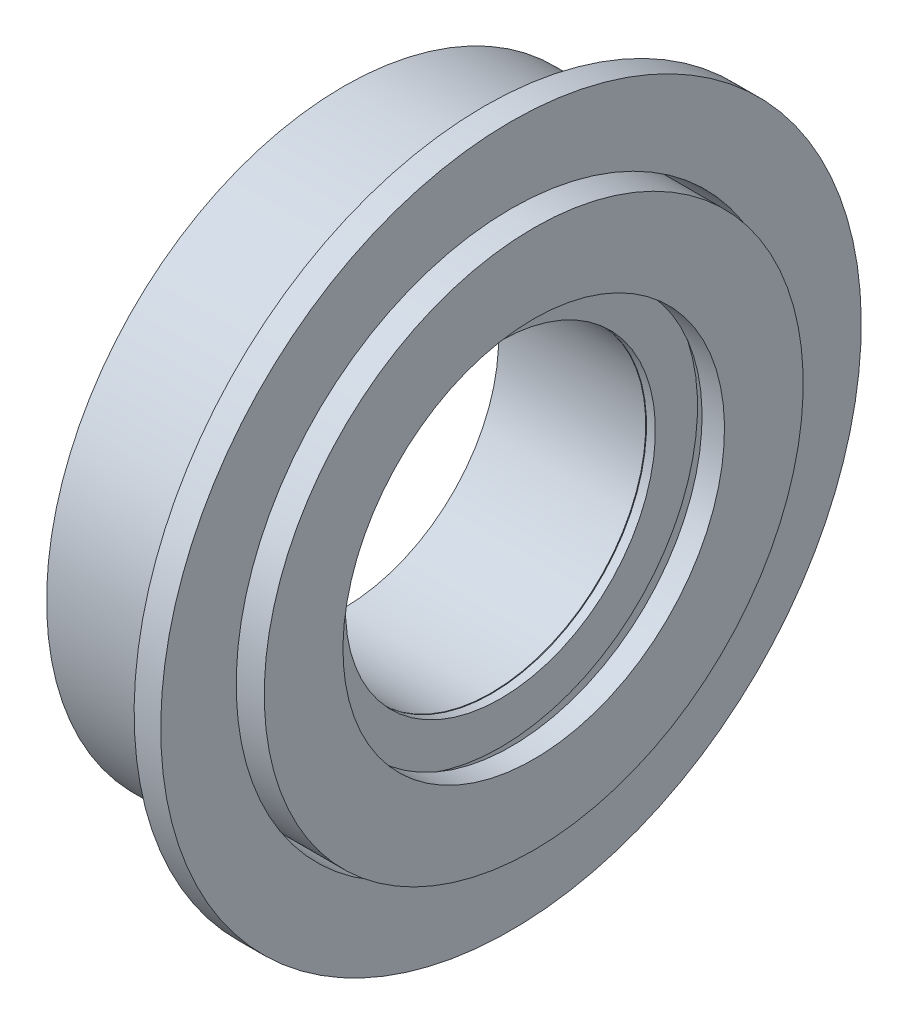
from build123d import *

# Parameters (mm, degrees)
SKETCH1_W   = 12.624761142
SKETCH1_H   = 6.080044682
SKETCH1_W_2 = 1
SKETCH1_H_2 = 4.744556516


with BuildPart() as part:
    # Sketch1 → Revolve1 (revolve)
    with BuildSketch(Plane.XY):
        Polygon((93, 39.45458405), (93, 33.45458405), (93, 30.95458405), (77, 30.95458405), (77, 20.45458405), (90.724333667, 20.45458405), (90.724333667, 17.45458405), (74.14259961, 17.45458405), (74.14259961, 33.45458405), (90, 33.45458405), (90, 39.45458405), align=None)
        Polygon((77.84816745, 30.355462664), (92, 30.355462664), (95.560954263, 30.355462664), (95.560954263, 21.489590566), (93.034479753, 21.489590566), (93.034479753, 25.002117737), (90.724333667, 25.002117737), (90.724333667, 26.574131723), (77.84816745, 26.574131723), align=None)
        with Locations((84.40932732, 23.531873601)):
            Rectangle(SKETCH1_W, SKETCH1_H)
        with Locations((91.311321069, 19.826862308)):
            Rectangle(SKETCH1_W_2, SKETCH1_H_2)
    revolve(axis=Axis((0, 0, 0), (-1, 0, 0)))


solid = part.part
